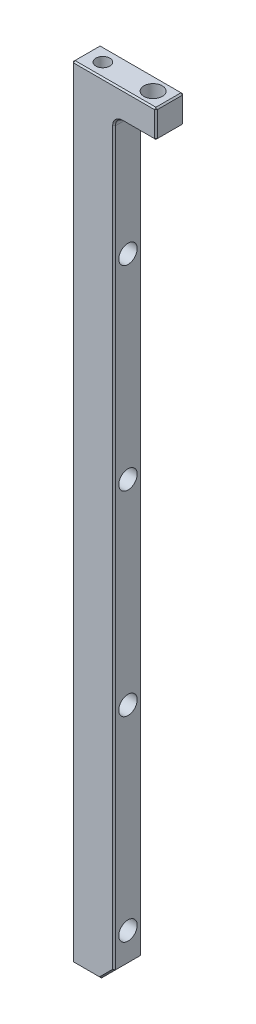
SolidWorks part; units mm, degrees
material "S45C"
ref_plane "前视基准面" through (0, 0, 0) normal (0, 0, 1) x (1, 0, 0)
ref_plane "上视基准面" through (0, 0, 0) normal (0, 1, 0) x (1, 0, 0)
ref_plane "右视基准面" through (0, 0, 0) normal (1, 0, 0) x (0, 0, -1)
sketch "草图1" plane through (0, 0, 0) normal (0, 0, 1) x (1, 0, 0)
  line L1 (-15, -140) -> (15, -140)
  line L2 (-15, -140) -> (-15, 140)
  line L3 (-15, 140) -> (15, 140)
  line L4 (15, -140) -> (15, 140)
  line L5 (-15, -140) -> (15, 140) construction
  line L6 (-15, 140) -> (15, -140) construction
  point P0 (0, 0)
  dimension "D1" = 30
  dimension "D2" = 280
extrude "凸台-拉伸1" add sketch "草图1" along normal mid plane 10
sketch "草图2" plane through (0, 0, -5) normal (0, 0, -1) x (-1, 0, 0)
  line L0 (-15, 140) -> (15, 140) construction
  line L1 (-15, -140) -> (0, -140)
  line L2 (-15, -140) -> (-15, 130)
  line L3 (-15, 130) -> (0, 130)
  line L4 (0, -140) -> (0, 130)
  dimension "D1" = 10
  dimension "D2" = 15
extrude "切除-拉伸1" cut sketch "草图2" against normal through all
fillet "圆角1" radius 3 1 edges at (0, 130, 0)
sketch "草图3" plane through (0, 130, 0) normal (0, -1, 0) x (-1, 0, 0)
  line L0 (-15, 0) -> (15, 0) construction
  line L1 (-15, -5) -> (-15, 5) construction
  line L2 (15, -5) -> (15, 5) construction
  point P0 (-9, 0)
  dimension "D1" = 6
hole_wizard "M6 间隙孔1" positions "草图3" profile "草图4" hole size "M6" standard "GB" end condition through all
sketch "草图4" plane through (9, 130, 0) normal (1, 0, 0) x (0, 0, -1)
  line L0 (0, 0) -> (0, 10)
  line L1 (0, 10) -> (3.3, 10)
  line L2 (3.3, 10) -> (3.3, 0)
  line L5 (3.3, 0) -> (0, 0)
  line L11 (0, -6.35) -> (0, 107.95) construction
  dimension "通孔孔直径" = 6.6
  dimension "通孔孔深度" = 10
chamfer "倒角1" distance 5 angle 45 1 edges at (0, -140, 0)
sketch "草图5" plane through (0, 0, 0) normal (1, 0, 0) x (0, 0, -1)
  line L1 (-5, 140) -> (5, 140) construction
  line L3 (0, 85) -> (0, 15) construction
  line L4 (0, 15) -> (0, -55) construction
  line L5 (0, -55) -> (0, -125) construction
  line L11 (5, -140) -> (-5, -140) construction
  point P0 (0, 85)
  point P2 (0, 15)
  point P4 (0, -55)
  point P19 (0, -125)
  dimension "D1" = 55
  dimension "D2" = 15
hole_wizard "M6 间隙孔2" positions "草图5" profile "草图6" hole size "M6" standard "GB" end condition through all
sketch "草图6" plane through (0, 85, 0) normal (0, 1, 0) x (0, 0, -1)
  line L0 (0, 0) -> (0, 15)
  line L1 (0, 15) -> (3.3, 15)
  line L2 (3.3, 15) -> (3.3, 0)
  line L5 (3.3, 0) -> (0, 0)
  line L11 (0, -6.35) -> (0, 107.95) construction
  dimension "通孔孔直径" = 6.6
  dimension "通孔孔深度" = 15
chamfer "倒角2" distance 0.5 angle 45 20 edges at (-15, 0, 5) (0, 140, 5) (9, 130, 5) (0.8787, 129.1213, 5) (0, -4, 5) (-2.5, -137.5, 5) (-10, -140, 5) (0.8787, 129.1213, -5) (9, 130, -5) (15, 140, 0) (15, 135, 5) (15, 130, 0) (15, 135, -5) (0, 140, -5) (0, -4, -5) (-2.5, -137.5, -5) (-10, -140, -5) (-15, -140, 0) (-15, 0, -5) (-15, 140, 0)
sketch "草图7" plane through (0, 140, 0) normal (0, 1, 0) x (1, 0, 0)
  line L0 (9, 0) -> (-9, 0) construction
  point P0 (-9, 0)
  point P7 (9, 0)
  dimension "D1" = 18
hole_wizard "Ø5.0mm 暗销孔1" positions "草图7" profile "草图8" hole size "Ø5.0" standard "ISO"
sketch "草图8" plane through (-9, 140, 0) normal (1, 0, 0) x (0, 0, 1)
  line L0 (0, 0) -> (0, 7.5022)
  line L1 (0, 7.5022) -> (2.5, 6)
  line L2 (2.5, 6) -> (2.5, 0)
  line L5 (2.5, 0) -> (0, 0)
  line L10 (0, 7.5022) -> (-2.5, 6) construction
  line L11 (0, -6.35) -> (0, 107.95) construction
  dimension "孔直径" = 5
  dimension "孔深度" = 6
  dimension "导头角度" = 118
